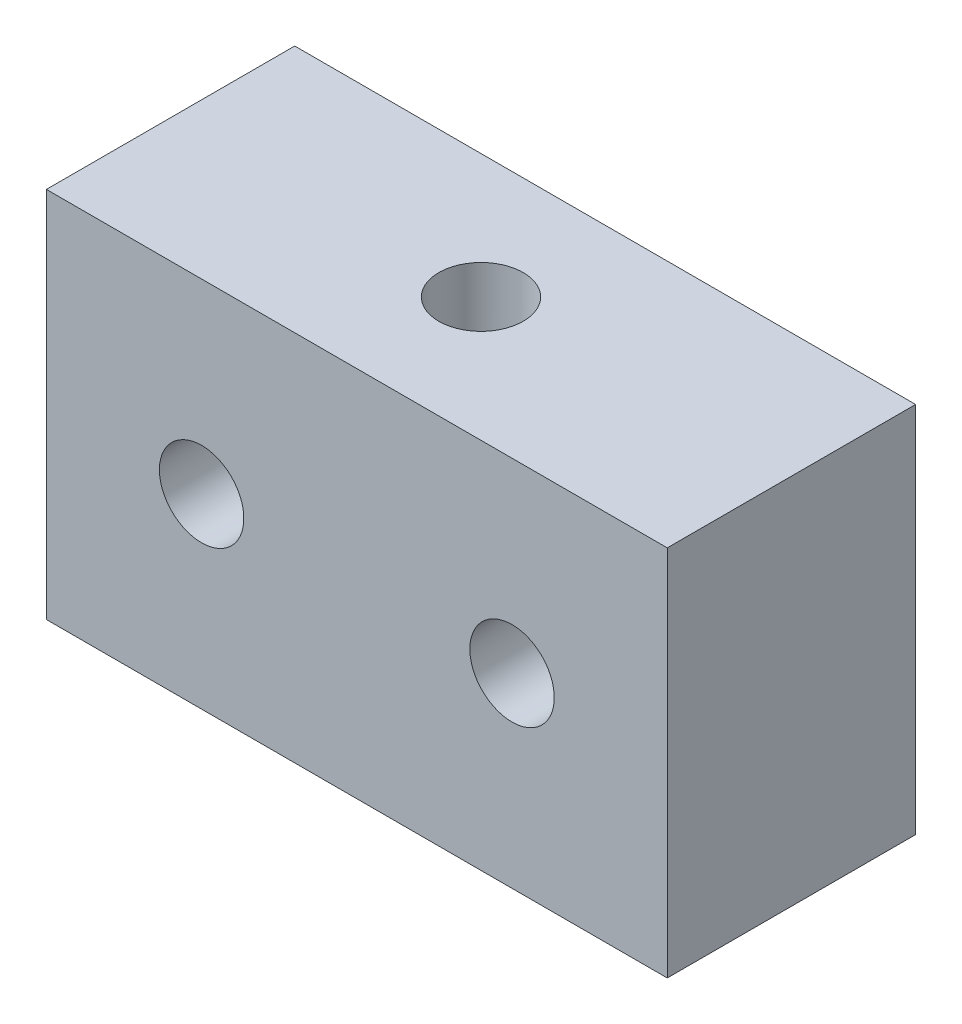
from build123d import *

# Parameters (mm, degrees)
SKETCH1_W           = 50
SKETCH1_H           = 30
BOSS_EXTRUDE1_DEPTH = 20
M8_TAPPED_HOLE1_D   = 6.8
M8_TAPPED_HOLE2_D   = 6.8
SKETCH6_R           = 4
CUT_EXTRUDE1_DEPTH  = 20


with BuildPart() as part:
    # Sketch1 → Boss-Extrude1 (new body)
    with BuildSketch(Plane.XY):
        with Locations((25, -15)):
            Rectangle(SKETCH1_W, SKETCH1_H)
    extrude(amount=BOSS_EXTRUDE1_DEPTH)

    # M8 Tapped Hole1 (through all)
    with Locations(Plane(origin=(0, 0, 0), x_dir=(-1, 0, 0), z_dir=(0, 0, -1))):
        with Locations((-12.5, -15), (-37.5, -15)):
            Hole(M8_TAPPED_HOLE1_D / 2)

    # M8 Tapped Hole2 (through all)
    with Locations(Plane(origin=(25, 0, 10), x_dir=(0, 0, 1), z_dir=(0, 1, 0))):
        with Locations((0, 0)):
            Hole(M8_TAPPED_HOLE2_D / 2)

    # Sketch6 → Cut-Extrude1 (cut)
    with BuildSketch(Plane.XZ.offset(30)):
        with Locations(Location((25, 10, 0), (0, 0, 270))):
            Circle(SKETCH6_R)
    extrude(amount=-CUT_EXTRUDE1_DEPTH, mode=Mode.SUBTRACT)


solid = part.part
